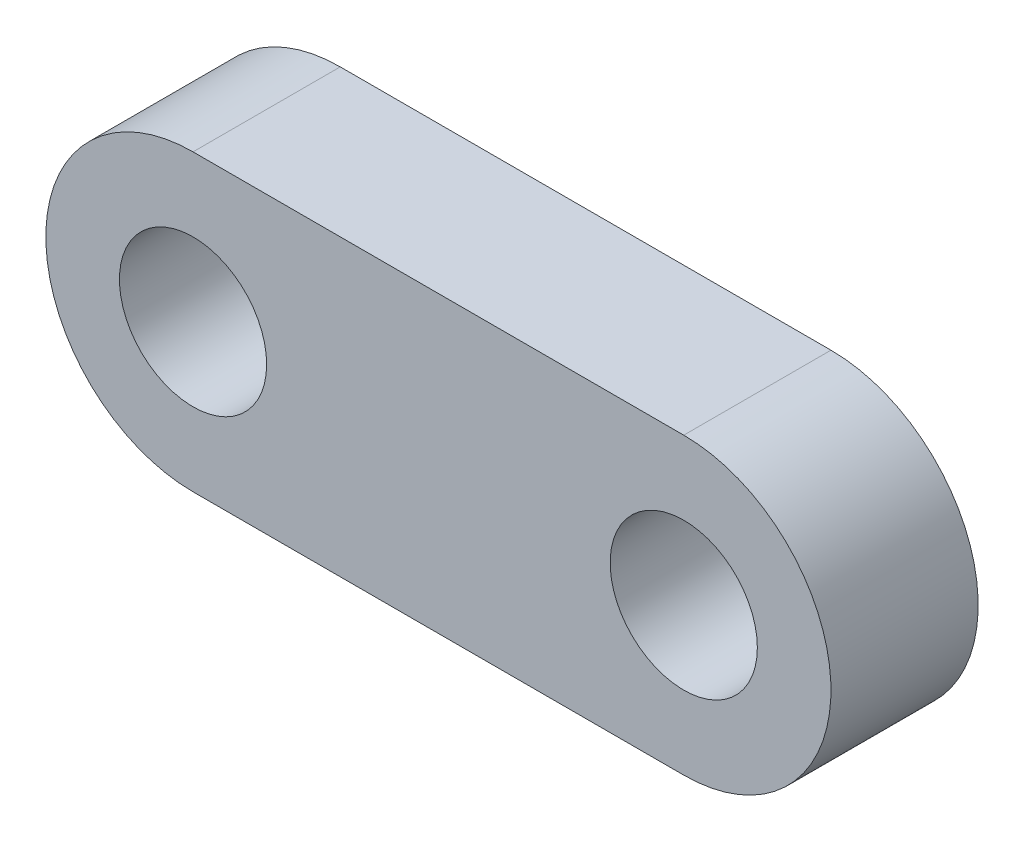
SolidWorks part; units mm, degrees
ref_plane "Front Plane" through (0, 0, 0) normal (0, 0, 1) x (1, 0, 0)
ref_plane "Top Plane" through (0, 0, 0) normal (0, 1, 0) x (1, 0, 0)
ref_plane "Right Plane" through (0, 0, 0) normal (1, 0, 0) x (0, 0, -1)
other "Configuration Table"
sketch "Sketch1" plane through (0, 0, 0) normal (0, 0, 1) x (1, 0, 0)
  line L0 (0, 0) -> (10, 0) construction
  line L1 (0, 3) -> (10, 3)
  line L2 (0, -3) -> (10, -3)
  arc A0 (0, 3) -> (0, -3) centre (0, 0) ccw
  arc A1 (10, -3) -> (10, 3) centre (10, 0) ccw
  circle A2 centre (0, 0) radius 1.5
  circle A3 centre (10, 0) radius 1.5
  point P3 (5, 0)
  dimension "D1" = 3
  dimension "D2" = 3
  dimension "D3" = 10
extrude "Boss-Extrude1" add sketch "Sketch1" along normal blind 3
